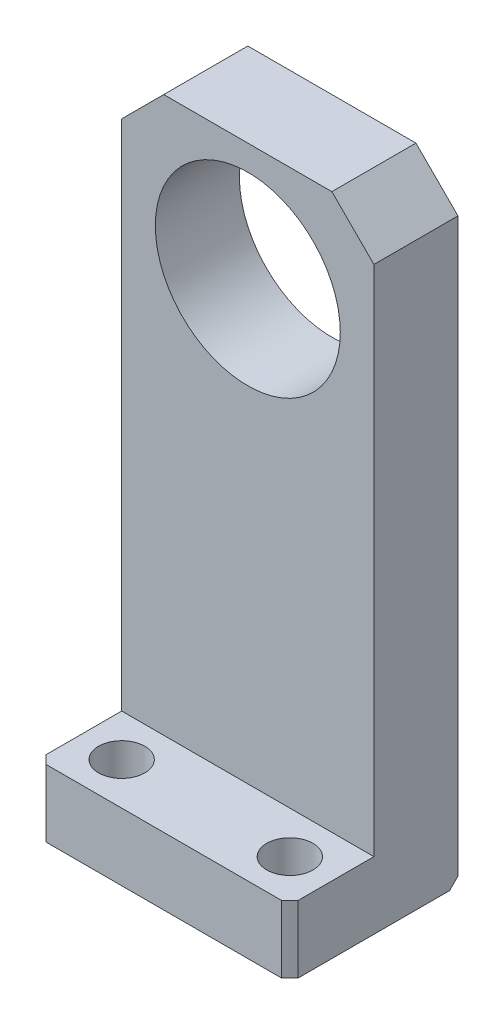
SolidWorks part; units mm, degrees
ref_plane "Front Plane" through (0, 0, 0) normal (0, 0, 1) x (1, 0, 0)
ref_plane "Top Plane" through (0, 0, 0) normal (0, 1, 0) x (1, 0, 0)
ref_plane "Right Plane" through (0, 0, 0) normal (1, 0, 0) x (0, 0, -1)
sketch "Sketch1" plane through (0, 0, 0) normal (0, 0, 1) x (1, 0, 0)
  line L0 (0, 0) -> (0, 74) construction
  line L1 (15, 0) -> (-15, 0)
  line L2 (15, 0) -> (15, 74)
  line L3 (15, 74) -> (-15, 74)
  line L4 (-15, 0) -> (-15, 74)
  circle A0 centre (0, 60) radius 11
  dimension "D1" = 22
  dimension "D2" = 60
  dimension "D3" = 74
  dimension "D4" = 30
extrude "Boss-Extrude1" add sketch "Sketch1" along normal blind 10
sketch "Sketch3" plane through (0, 0, 0) normal (0, -1, 0) x (1, 0, 0)
  line L0 (-15, 10) -> (-15, 20)
  line L1 (-15, 20) -> (0, 20)
  line L2 (0, 20) -> (0, 10)
  line L3 (-15, 10) -> (15, 10) construction
  line L4 (0, 0) -> (0, 20.2198) construction
  line L5 (0, 20) -> (0, 10)
  line L6 (15, 20) -> (0, 20)
  line L7 (15, 10) -> (15, 20)
  line M3 (15, 10) -> (-15, 10)
  dimension "D1" = 10
extrude "Boss-Extrude2" add sketch "Sketch3" against normal blind 8 contours L2 L1 L0 M3 | L7 L6 L5 M3
sketch "Sketch4" plane through (0, 8, 0) normal (0, 1, 0) x (-1, 0, 0)
  line L0 (0, 0) -> (0, 20.7183) construction
  line L1 (-15, 0) -> (15, 0) construction
  circle A0 centre (10, 15) radius 2.75
  circle A1 centre (-10, 15) radius 2.75
  dimension "D1" = 20
  dimension "D2" = 5.5
  dimension "D3" = 15
extrude "Cut-Extrude1" cut sketch "Sketch4" against normal through all
hole_wizard "Ø4.0 (4) Diameter Hole1" positions "Sketch7" profile "Sketch6" hole size "Ø4.0" standard "GB"
sketch "Sketch7" plane through (0, 0, 0) normal (0, -1, 0) x (1, 0, 0)
  line L0 (0, 0) -> (0, 13.6931) construction
  line L2 (-15, 0) -> (15, 0) construction
  point P0 (-10, 5)
  point P1 (10, 5)
  dimension "D1" = 20
  dimension "D2" = 5
sketch "Sketch6" plane through (-10, 0, 5) normal (1, 0, 0) x (0, 0, -1)
  line L0 (0, 0) -> (0, 11.2017)
  line L1 (0, 11.2017) -> (2, 10)
  line L2 (2, 10) -> (2, 0)
  line L5 (2, 0) -> (0, 0)
  line L10 (0, 11.2017) -> (-2, 10) construction
  line L11 (0, -6.35) -> (0, 107.95) construction
  dimension "孔直径" = 4
  dimension "孔深度" = 10
  dimension "导头角度" = 118
chamfer "Chamfer1" distance 5 angle 45 2 edges at (-15, 74, 5) (15, 74, 5)
chamfer "Chamfer2" distance 1 angle 45 3 edges at (-15, 4, 20) (15, 4, 20) (0, 0, 0)
